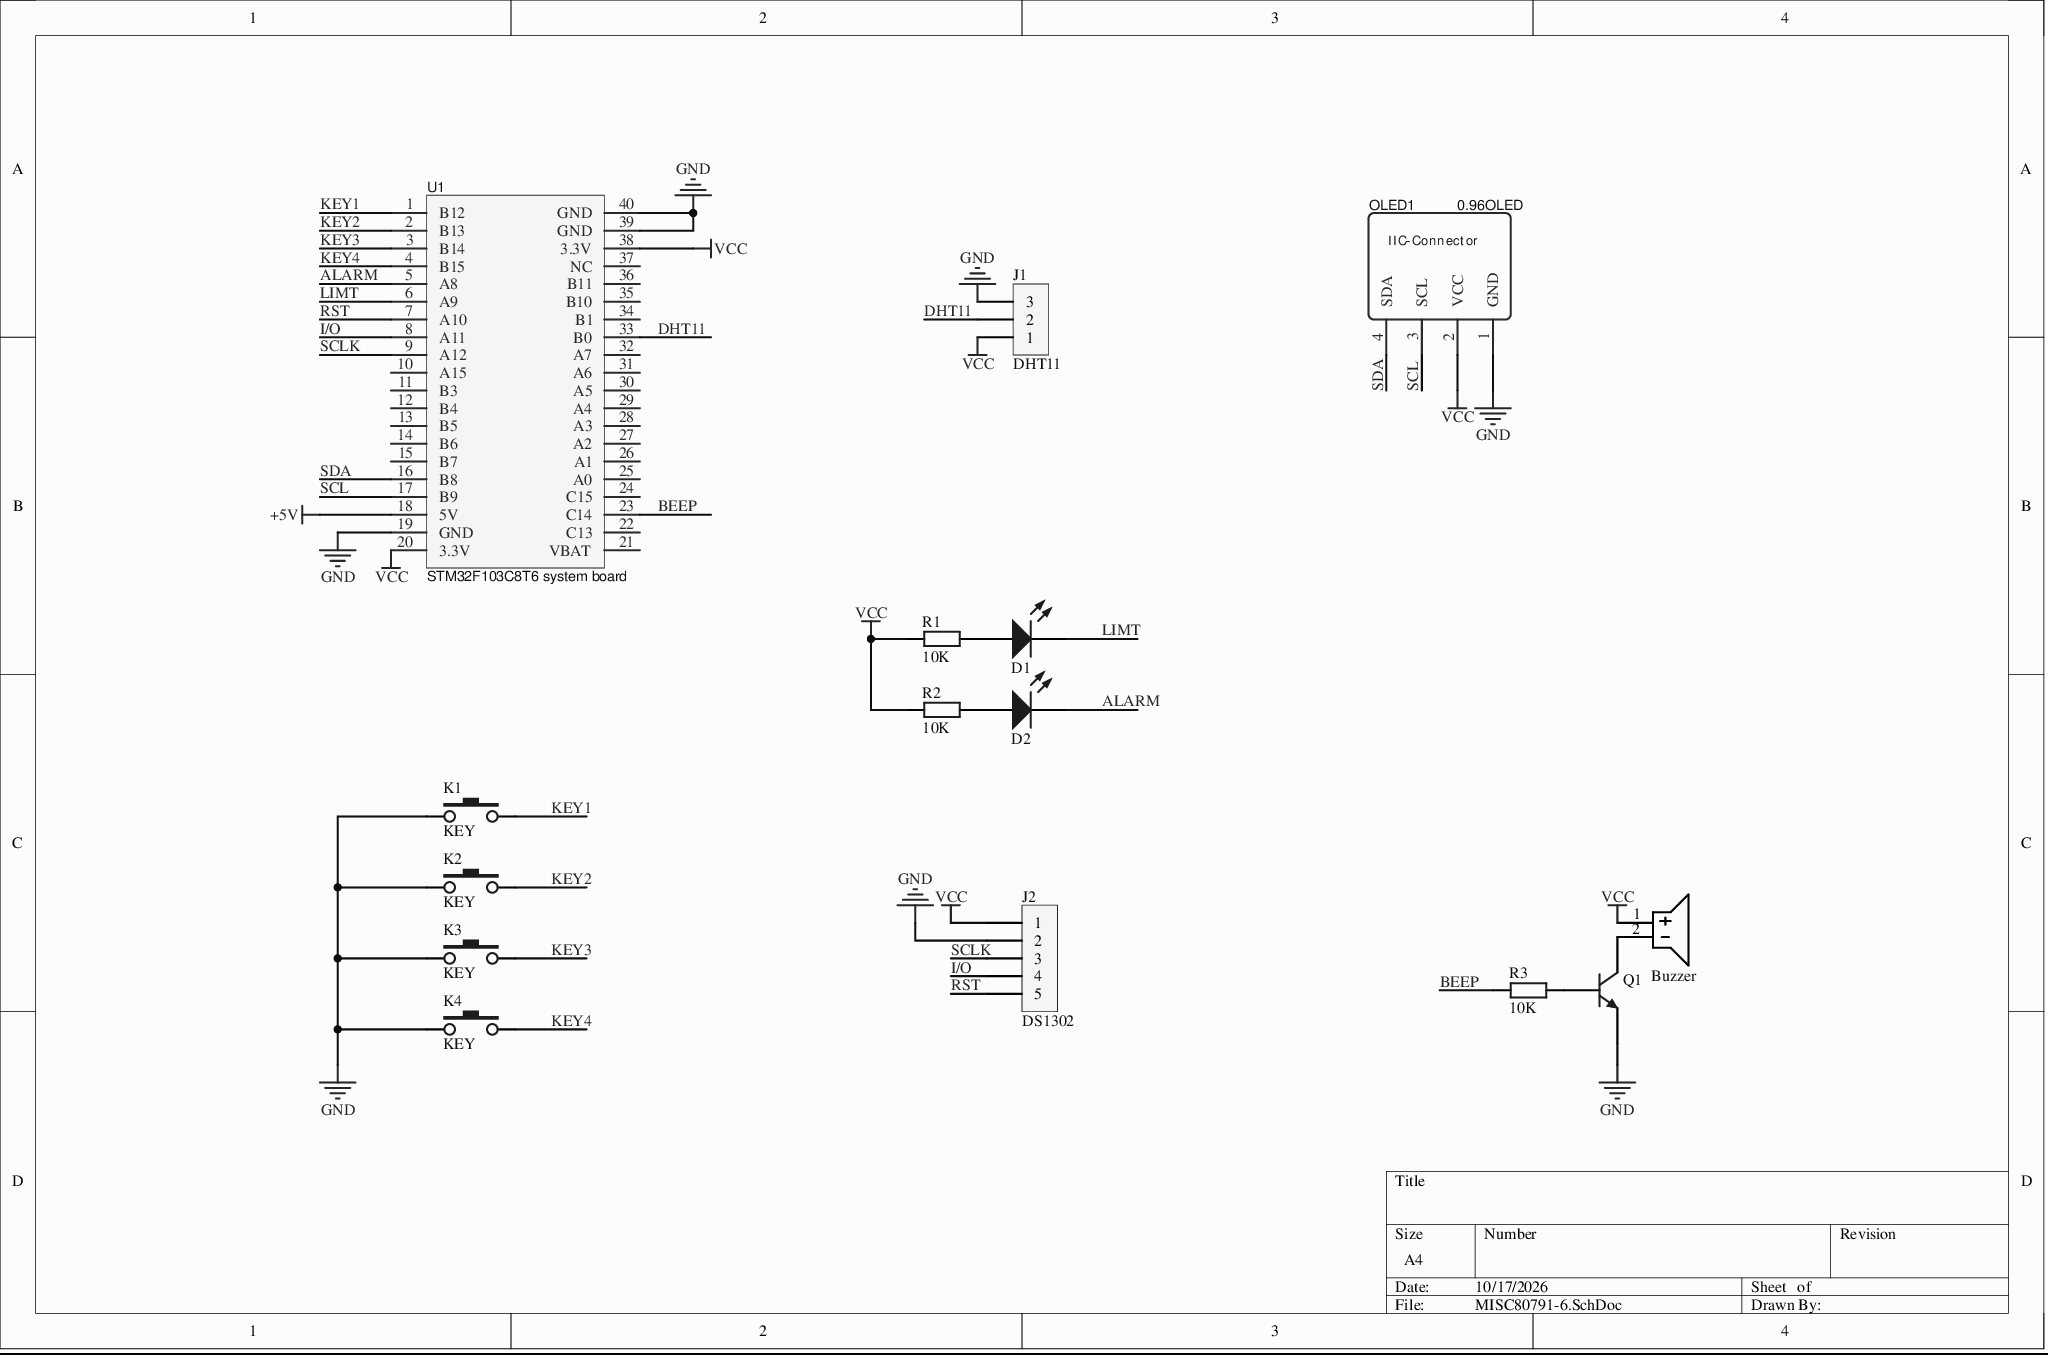
[diagram p0: MISC80791-6.SchDoc]
# Altium project MISC80791-2.PrjPcb
1 sheet, 15 parts. Net scope: global (net labels, ports and power ports of the same name join across sheets).
Board file: MISC80791.PcbDoc

## Sheet MISC80791-6.SchDoc
size A4

### Parts
*1  Buzzer  [BUZZER]
D1  LED  [LED 5MM-W]  (value not drawn)
D2  LED  [LED 5MM-W]  (value not drawn)
J1  DHT11  [Fe-HDR1X3/2.54-S]
J2  DS1302  [Fe-HDR1X5/2.54-S]
K1  KEY  [DIP-3X6X4.3]
K2  KEY  [DIP-3X6X4.3]
K3  KEY  [DIP-3X6X4.3]
K4  KEY  [DIP-3X6X4.3]
OLED1  0.96OLED  [0.96OLED_4P]
Q1  2N3904  [TO-92A]  (value not drawn)
R1  10K  [RS 1/4W]
R2  10K  [RS 1/4W]
R3  10K  [RS 1/4W]
U1  STM32F103C8T6 system board  [STM32核心板]

### Nets
+5V: U1.18(5V)
GND: J1.3 J2.2 K1.1 K2.1 K3.1 K4.1 OLED1.1(GND) Q1.1(E) U1.19(GND) U1.39(GND) U1.40(GND)
VCC: *1.1 J1.1 J2.1 OLED1.2(VCC) R1.1 R2.1 U1.20(3.3V) U1.38(3.3V)
ALARM: D2.2(K) U1.5(A8)
BEEP: R3.1 U1.23(C14)
DHT11: J1.2 U1.33(B0)
I/O: J2.4 U1.8(A11)
KEY1: K1.3 U1.1(B12)
KEY2: K2.3 U1.2(B13)
KEY3: K3.3 U1.3(B14)
KEY4: K4.3 U1.4(B15)
LIMT: D1.2(K) U1.6(A9)
RST: J2.5 U1.7(A10)
SCL: OLED1.3(SCL) U1.17(B9)
SCLK: J2.3 U1.9(A12)
SDA: OLED1.4(SDA) U1.16(B8)
Net*1_2: *1.2 Q1.3(C)
NetD1_1: D1.1(A) R1.2
NetD2_1: D2.1(A) R2.2
NetQ1_2: Q1.2(B) R3.2

Not connected (* = marked no-connect by the designer): U1 10(A15) 11(B3) 12(B4) 13(B5) 14(B6) 15(B7) 21(VBAT) 22(C13) 24(C15) 25(A0) 26(A1) 27(A2) 28(A3) 29(A4) 30(A5) 31(A6) 32(A7) 34(B1) 35(B10) 36(B11) 37(NC)

### Library data of the parts
D1 D2 = LED: Light-emitting diode
J1 = Female HDR1X3
J2 = Female HDR1X5
OLED1 = 0.96OLED_4P_MODULE_JX: Manufacturer: null; Contributor: LCSC; Supplier: LCSC; Supplier Part: C9900004566; Manufacturer Part: 0.96OLED_4P_MODULE_JX; JLCPCB Part Class: Extended Part; link: https://so.szlcsc.com/global.html?k=C9900004566&ref=editor; spicePre: O; spiceSymbolName: 0.96OLED_4P_MODULE_JX
Q1 = 2N3904: NPN General Purpose Amplifier; Published: 8-Jun-2000; LatestRevisionDate: 15-Jan-2003; LatestRevisionNote: PCB Footprint 'BCY-W3/D4.7' replaced; DatasheetVersion: 1997; PackageVersion: Sep-1998; PackageReference: TO-92A; PackageDescription: TO, Flat Index; 3 In-Line, Axial Leads; Body Dia. 4.5mm; Leads 0.51 x 0.48 mm (max); ComponentLink1Description: Manufacturer Link; ComponentLink2Description: Datasheet; ComponentLink2URL: http://www.fairchildsemi.com/ds/2N%2F2N3904.pdf; Publisher: Altium Limited
R1-R3 = R-S: Color-band resistor; BOM名称: Color-band resistor
U1 = STM32F103C8T6系统板: Contributor: wwwxxb; spicePre: U; spiceSymbolName: STM32F103C8T6 system board